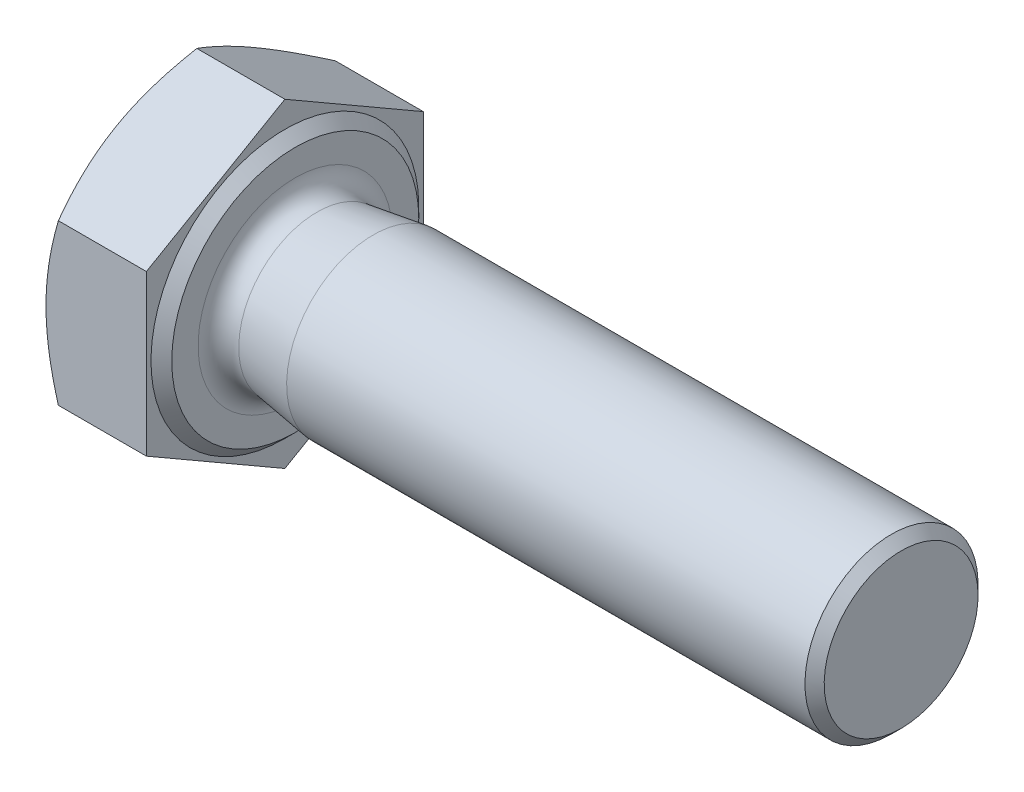
SolidWorks part; units mm, degrees
ref_plane "前视基准面" through (0, 0, 0) normal (0, 0, 1) x (1, 0, 0)
ref_plane "上视基准面" through (0, 0, 0) normal (0, 1, 0) x (1, 0, 0)
ref_plane "右视基准面" through (0, 0, 0) normal (1, 0, 0) x (0, 0, -1)
sketch "草图1" plane through (0, 0, 0) normal (0, 0, 1) x (1, 0, 0)
  line L0 (0, 0) -> (41.4, 0) construction
  line L1 (0, 0) -> (0, 8.795)
  line L2 (0, 8.795) -> (6.4, 8.795)
  line L3 (6.4, 8.795) -> (6.4, 0)
  line L4 (6.4, 5) -> (41.4, 5)
  line L5 (41.4, 5) -> (41.4, 0)
  line L6 (0, 8) -> (0.459, 8.795)
  line L7 (38.4, 5) -> (38.4, 0)
  line L8 (10.9, 5) -> (10.9, 0)
  line L9 (6.4, 4.5129) -> (41.4, 4.5129)
  line L10 (41.4, 4.1881) -> (6.4, 4.1881)
  line L11 (5.8, 7.735) -> (6.4, 7.135)
  line L12 (5.8, 8.795) -> (5.8, 0)
  line L13 (6.3, 7.235) -> (6.3, 0) construction
  arc A0 (6.4, 6.1) -> (7.5, 5) centre (7.5, 6.1) ccw
  point P12 (39.9, 0)
  point P13 (2.23, 8.795)
  point P14 (6.4, 6.1)
  point P24 (6.4, 7.235)
  dimension "D1" = 0.1
  dimension "r" = 1.1
  dimension "k" = 6.4
  dimension "D2" = 45
  dimension "β" = 30
  dimension "e" = 17.59
  dimension "s" = 16
  dimension "d" = 10
  dimension "l" = 35
  dimension "D52" = 3
  dimension "P" = 1.5
  dimension "kw" = 4.17
  dimension "da" = 12.2
  dimension "a" = 4.5
  dimension "ds" = 9.0258
  dimension "D61" = 8.3763
  dimension "dw" = 14.47
  dimension "c" = 0.6
sketch "草图2" plane through (0, 0, 0) normal (1, 0, 0) x (0, 0, -1)
  line L1 (0, 9.2376) -> (-8, 4.6188)
  line L2 (-8, 4.6188) -> (-8, -4.6188)
  line L3 (-8, -4.6188) -> (0, -9.2376)
  line L4 (0, -9.2376) -> (8, -4.6188)
  line L5 (8, -4.6188) -> (8, 4.6188)
  line L6 (8, 4.6188) -> (0, 9.2376)
  circle A0 centre (0, 0) radius 8 construction
sketch "草图3" plane through (0, 0, 0) normal (1, 0, 0) x (0, 0, -1)
  line L0 (8, 4.6188) -> (0, 9.2376) construction
  line L1 (0, 9.2376) -> (-8, 4.6188) construction
  line L2 (-8, 4.6188) -> (-8, -4.6188) construction
  line L3 (8, -4.6188) -> (8, 4.6188) construction
  line L4 (0, -9.2376) -> (8, -4.6188) construction
  line L5 (-8, -4.6188) -> (0, -9.2376) construction
  line L6 (8, 4.6188) -> (0, 9.2376)
  line L7 (0, 9.2376) -> (-8, 4.6188)
  line L8 (-8, 4.6188) -> (-8, -4.6188)
  line L9 (8, -4.6188) -> (8, 4.6188)
  line L10 (0, -9.2376) -> (8, -4.6188)
  line L11 (-8, -4.6188) -> (0, -9.2376)
extrude "凸台-拉伸1" add sketch "草图3" along normal up to vertex (6.4 mm away) up to point (6.4, 8.795, 0)
sketch "草图4" plane through (0, 0, 0) normal (-1, 0, 0) x (0, 0, 1)
  circle A0 centre (0, 0) radius 8 construction
  circle A1 centre (0, 0) radius 8
  circle A2 centre (0, 0) radius 17.59
  dimension "D1" = 35.18
extrude "切除-拉伸1" cut sketch "草图4" against normal blind 0.8 draft 60
sketch "草图5" [suppressed] plane through (0, 0, 0) normal (0, 0, 1) x (1, 0, 0)
  line L0 (35, 28) -> (100, 28) construction
  line L1 (100, 28) -> (100, 0) construction
  line L2 (0, 0) -> (100, 0) construction
  line L3 (40.5, 28) -> (100, 28)
  line L4 (100, 28) -> (100, 0)
  line L5 (35, 0) -> (100, 0)
  line L6 (35, 33.5) -> (35, 0)
  arc A0 (35, 33.5) -> (40.5, 28) centre (40.5, 33.5) ccw construction
  arc A1 (35, 33.5) -> (40.5, 28) centre (40.5, 33.5) ccw
revolve "旋转1" add sketch "草图5" angle 360 about L5
cosmetic thread "装饰螺纹线2" [suppressed] parameters "D1"=30.5, "D2"=8.3763
chamfer "倒角2" [suppressed] distance 0.5556 angle 45
sketch "草图7" plane through (0, 0, 0) normal (0, 0, 1) x (1, 0, 0)
  line L0 (6.4, 7.135) -> (5.8, 7.735)
  line L1 (5.8, 7.735) -> (5.8, 17.59)
  line L2 (5.8, 17.59) -> (6.4, 17.59)
  line L3 (6.4, 17.59) -> (6.4, 7.135)
  line L4 (0, 0) -> (41.4, 0) construction
  line L5 (0, 0) -> (41.4, 0) construction
  dimension "D1" = 35.18
revolve "切除-旋转1" [suppressed] cut sketch "草图7" angle 360 mid plane about L5
sketch "草图6" plane through (0, 0, 0) normal (0, 0, 1) x (1, 0, 0)
  line L0 (10.9, 0) -> (10.9, 5) construction
  line L1 (10.9, 5) -> (41.4, 5)
  line L2 (41.4, 5) -> (41.4, 0)
  line L3 (10.9, 5) -> (7.6597, 4.5245)
  line L5 (6.4, 4.5129) -> (41.4, 4.5129) construction
  line L6 (6.4, 8.795) -> (6.4, 0) construction
  line L7 (6.4, 5.6129) -> (6.4, 0)
  line L8 (6.4, 0) -> (41.4, 0)
  arc A0 (7.6597, 4.5245) -> (6.4, 5.6129) centre (7.5, 5.6129) cw
  arc A1 (6.4, 6.1) -> (7.5, 5) centre (7.5, 6.1) ccw construction
revolve "旋转2" add sketch "草图6" angle 360 about L8
cosmetic thread "装饰螺纹线1" parameters "D1"=30.5, "D2"=8.3763
chamfer "倒角1" distance 0.5556 angle 45 1 edges at (41.4, -5, 0)
sketch "草图8" plane through (0, 0, 0) normal (0, 0, 1) x (1, 0, 0)
  line L0 (6.4, 7.135) -> (5.8, 7.735)
  line L1 (5.8, 7.735) -> (5.8, 17.59)
  line L2 (5.8, 17.59) -> (6.4, 17.59)
  line L3 (6.4, 17.59) -> (6.4, 7.135)
  line L4 (0, 0) -> (41.4, 0) construction
  line L5 (0, 0) -> (41.4, 0) construction
  dimension "D1" = 35.18
revolve "切除-旋转2" cut sketch "草图8" angle 360 mid plane about L5
